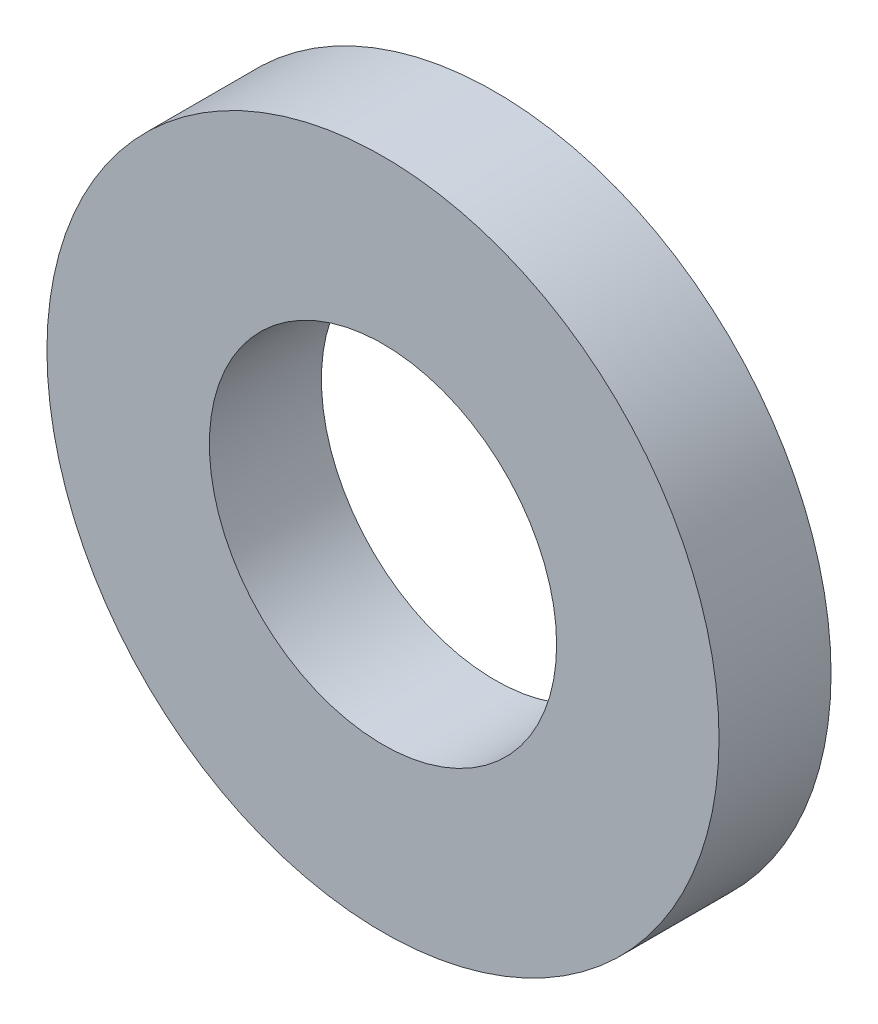
SolidWorks part; units mm, degrees
material "SUS304"
ref_plane "前视基准面" through (0, 0, 0) normal (0, 0, 1) x (1, 0, 0)
ref_plane "上视基准面" through (0, 0, 0) normal (0, 1, 0) x (1, 0, 0)
ref_plane "右视基准面" through (0, 0, 0) normal (1, 0, 0) x (0, 0, -1)
sketch "Sketch1" plane through (0, 0, 0) normal (0, 0, 1) x (1, 0, 0)
  circle A0 centre (0, 0) radius 3.1
  circle A1 centre (0, 0) radius 6
  dimension "D1" = 12
  dimension "D2" = 6.2
extrude "Extrude1" add sketch "Sketch1" along normal blind 2
